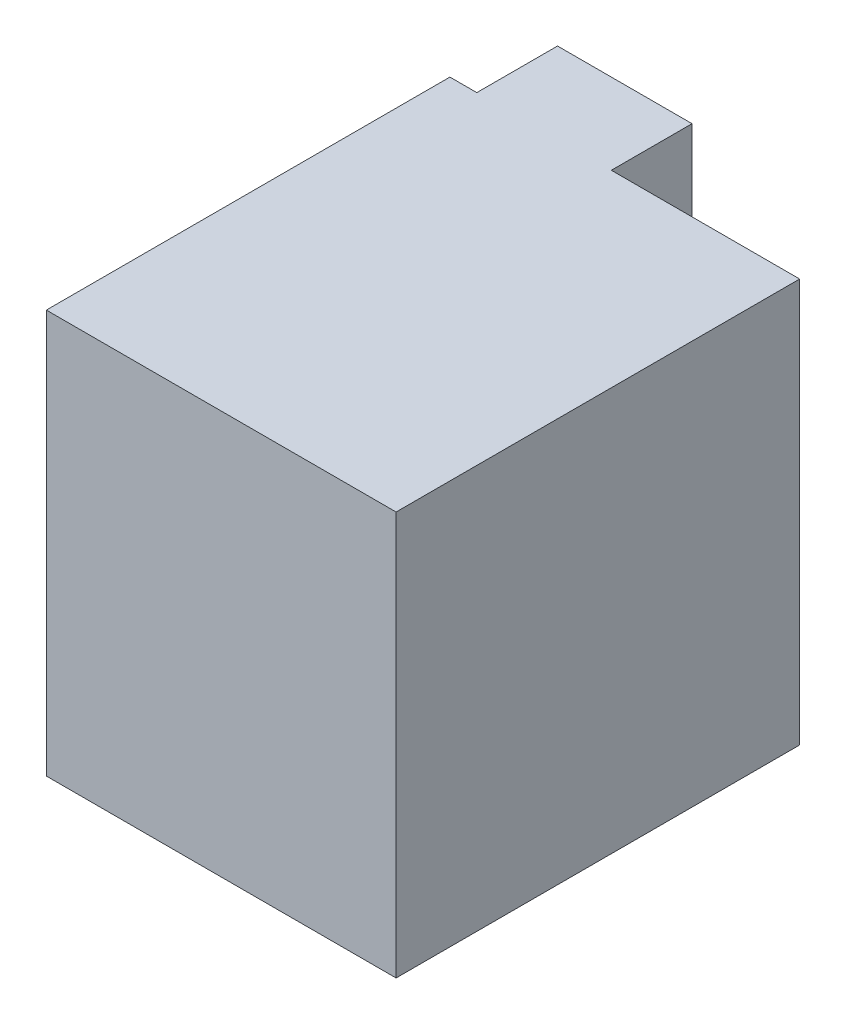
from build123d import *

# Parameters (mm, degrees)
EXTRUDE_1_DEPTH = 150


with BuildPart() as part:
    # 草图1 → 凸台-拉伸1 (new body)
    with BuildSketch(Plane(origin=(0, 0, 0), x_dir=(1, 0, 0), z_dir=(0, 1, 0))):
        Polygon((0, 0), (130, 0), (130, 150), (60, 150), (60, 180), (10, 180), (10, 150), (0, 150), align=None)
    extrude(amount=EXTRUDE_1_DEPTH)


solid = part.part
